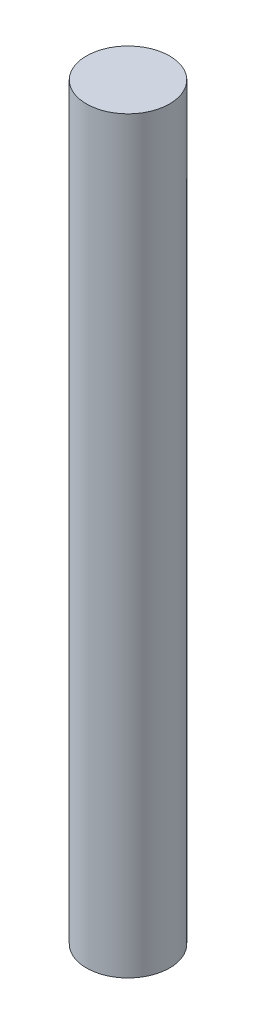
SolidWorks part; units mm, degrees
ref_plane "Front Plane" through (0, 0, 0) normal (0, 0, 1) x (1, 0, 0)
ref_plane "Top Plane" through (0, 0, 0) normal (0, 1, 0) x (1, 0, 0)
ref_plane "Right Plane" through (0, 0, 0) normal (1, 0, 0) x (0, 0, -1)
other "Configuration Table"
sketch "Sketch1" plane through (0, 0, 0) normal (0, 1, 0) x (1, 0, 0)
  circle A0 centre (0, 0) radius 10
  dimension "D1" = 20
extrude "Boss-Extrude1" add sketch "Sketch1" along normal blind 180
cosmetic thread "Cosmetic Thread1"
